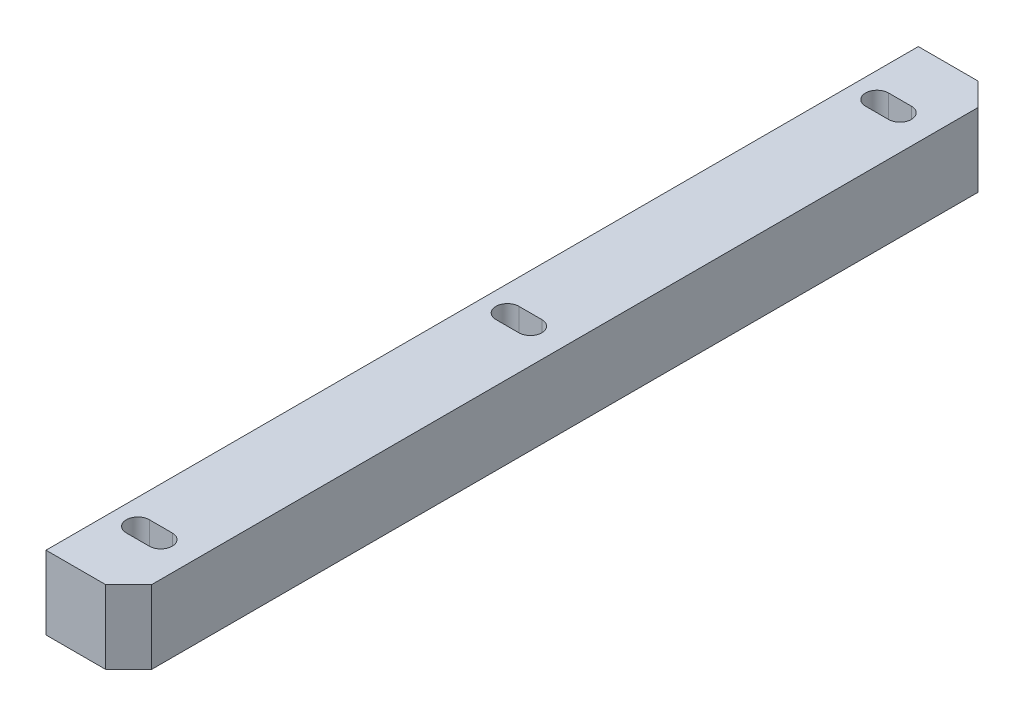
SolidWorks part; units mm, degrees
ref_plane "前视基准面" through (0, 0, 0) normal (0, 0, 1) x (1, 0, 0)
ref_plane "上视基准面" through (0, 0, 0) normal (0, 1, 0) x (1, 0, 0)
ref_plane "右视基准面" through (0, 0, 0) normal (1, 0, 0) x (0, 0, -1)
sketch "草图1" plane through (0, 0, 0) normal (0, 0, 1) x (1, 0, 0)
  line L0 (0, 0) -> (0, 16)
  line L1 (0, 16) -> (18, 16)
  line L4 (18, 16) -> (18, 0)
  line L5 (18, 0) -> (0, 0)
  dimension "D1" = 16
  dimension "D4" = 18
extrude "凸台-拉伸1" add sketch "草图1" along normal mid plane 190
chamfer "倒角1" distance 5 angle 45 2 edges at (18, 8, -95) (18, 8, 95)
sketch "草图2" plane through (0, 0, 0) normal (0, -1, 0) x (1, 0, 0)
  line L0 (5.5, 80.5) -> (10.5, 80.5) construction
  line L1 (5.5, 83) -> (10.5, 83)
  line L2 (5.5, 78) -> (10.5, 78)
  line L3 (0, 95) -> (0, -95) construction
  line L4 (0, 95) -> (13, 95) construction
  line L5 (5.5, 0) -> (10.5, 0) construction
  line L6 (5.5, 2.5) -> (10.5, 2.5)
  line L7 (5.5, -2.5) -> (10.5, -2.5)
  line L8 (0, -95) -> (13, -95) construction
  line L10 (5.5, -80.5) -> (10.5, -80.5) construction
  line L11 (5.5, -83) -> (10.5, -83)
  line L12 (5.5, -78) -> (10.5, -78)
  arc A0 (5.5, 83) -> (5.5, 78) centre (5.5, 80.5) ccw
  arc A1 (10.5, 78) -> (10.5, 83) centre (10.5, 80.5) ccw
  arc A2 (5.5, 2.5) -> (5.5, -2.5) centre (5.5, 0) ccw
  arc A3 (10.5, -2.5) -> (10.5, 2.5) centre (10.5, 0) ccw
  arc A4 (5.5, -83) -> (5.5, -78) centre (5.5, -80.5) cw
  arc A5 (10.5, -78) -> (10.5, -83) centre (10.5, -80.5) cw
  point P2 (8, 80.5)
  point P13 (8, 0)
  point P25 (8, -80.5)
  dimension "D1" = 2.5
  dimension "D2" = 5
  dimension "D3" = 8
  dimension "D4" = 12
  dimension "D5" = 5
  dimension "D6" = 12
extrude "切除-拉伸1" cut sketch "草图2" against normal up to next
